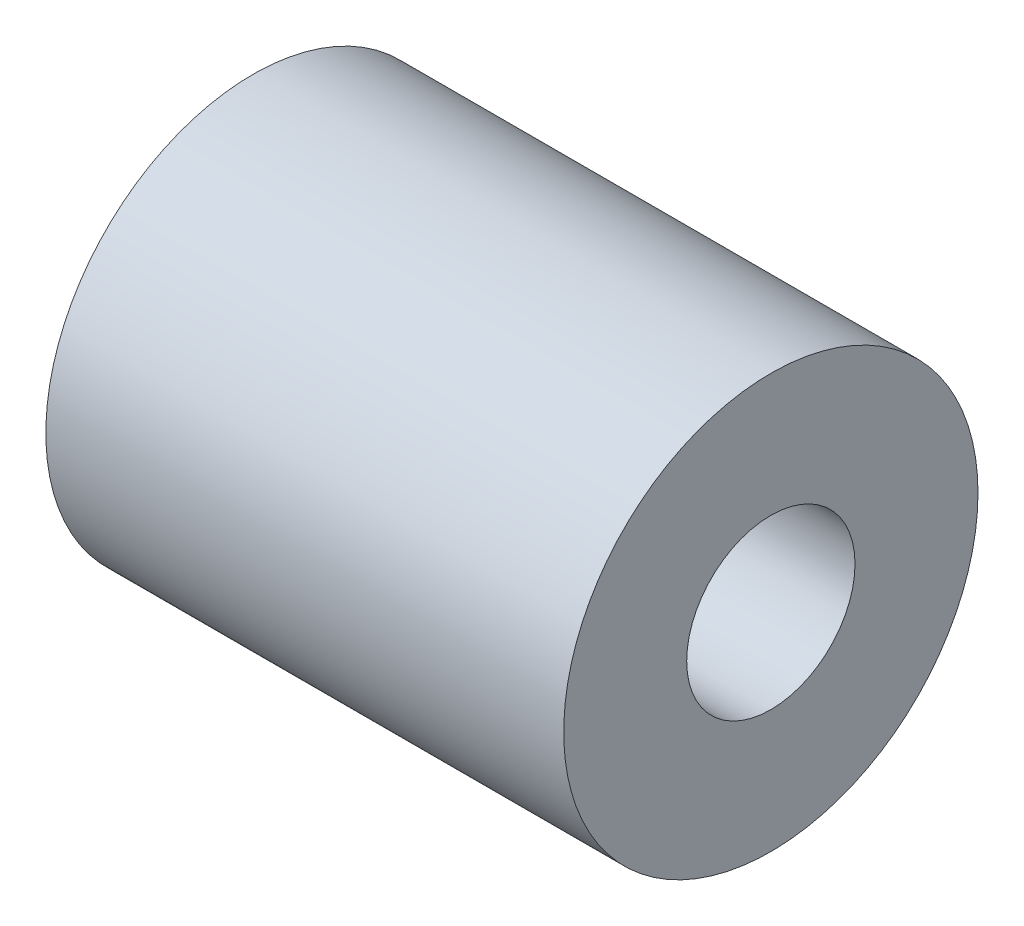
SolidWorks part; units mm, degrees
material "PP"
ref_plane "前视基准面" through (0, 0, 0) normal (0, 0, 1) x (1, 0, 0)
ref_plane "上视基准面" through (0, 0, 0) normal (0, 1, 0) x (1, 0, 0)
ref_plane "右视基准面" through (0, 0, 0) normal (1, 0, 0) x (0, 0, -1)
sketch "草图1" plane through (0, 0, 0) normal (1, 0, 0) x (0, 0, -1)
  circle A0 centre (0, 0) radius 8
  circle A1 centre (0, 0) radius 3.25
  dimension "D1" = 6.5
  dimension "D2" = 16
extrude "凸台-拉伸1" add sketch "草图1" along normal blind 20
